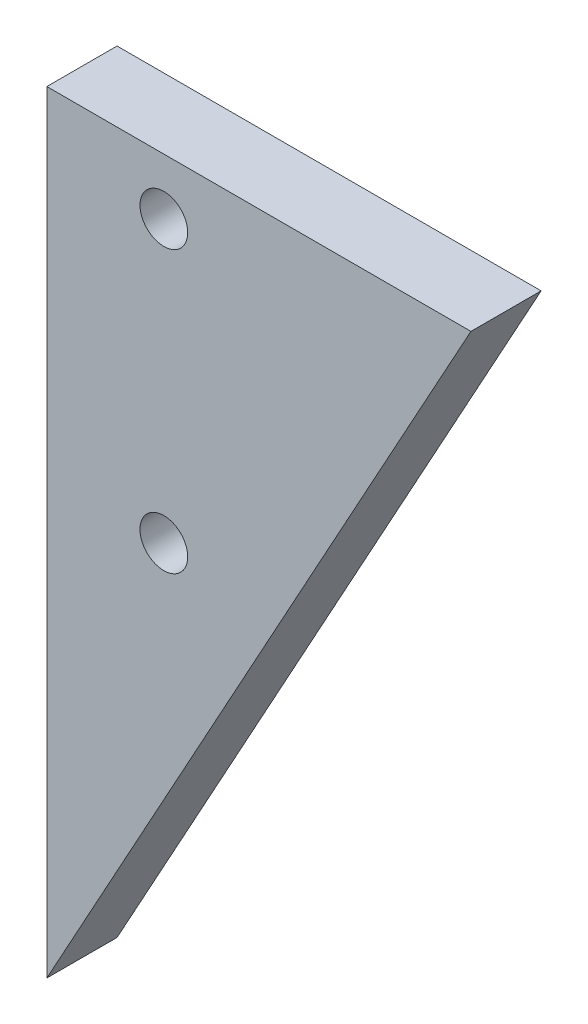
from build123d import *

# Parameters (mm, degrees)
SKETCH1_R              = 4.5
BOSS_EXTRUDE2_DEPTH    = 15
M12_TAPPED_HOLE1_D     = 10.2
M12_TAPPED_HOLE1_DEPTH = 29.25
M12_TAPPED_HOLE1_TIP   = 3.064389157


with BuildPart() as part:
    # Sketch1 → Boss-Extrude2 (new body)
    with BuildSketch(Plane.XY):
        Polygon((0, 0), (-90.634528925, 0), (-90.634528925, -165), align=None)
        with Locations((-65.634528925, -12)):
            Circle(SKETCH1_R, mode=Mode.SUBTRACT)
        with Locations((-65.634528925, -72)):
            Circle(SKETCH1_R, mode=Mode.SUBTRACT)
    extrude(amount=BOSS_EXTRUDE2_DEPTH)

    # M12 Tapped Hole1
    with Locations(Plane.XY.offset(15)):
        with Locations((-65.634528925, -12), (-65.634528925, -72)):
            Hole(M12_TAPPED_HOLE1_D / 2, depth=M12_TAPPED_HOLE1_DEPTH)
            with Locations((0, 0, -(M12_TAPPED_HOLE1_DEPTH + M12_TAPPED_HOLE1_TIP / 2))):  # 118° drill point
                Cone(0, M12_TAPPED_HOLE1_D / 2, M12_TAPPED_HOLE1_TIP, mode=Mode.SUBTRACT)


solid = part.part
